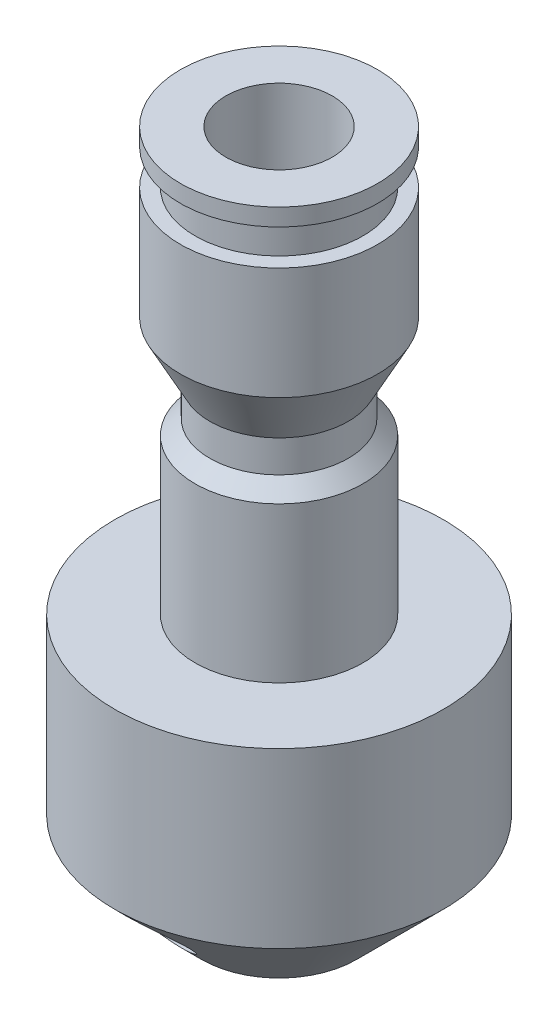
SolidWorks part; units mm, degrees
ref_plane "Front Plane" through (0, 0, 0) normal (0, 0, 1) x (1, 0, 0)
ref_plane "Top Plane" through (0, 0, 0) normal (0, 1, 0) x (1, 0, 0)
ref_plane "Right Plane" through (0, 0, 0) normal (1, 0, 0) x (0, 0, -1)
other "Configuration Table"
sketch "Sketch1" plane through (0, 0, 0) normal (0, 0, 1) x (1, 0, 0)
  line L2 (-8.5, -6.487) -> (-8.5, -9.5097) construction
  line L3 (-4.3412, -6.487) -> (-8.5, -6.487) construction
  line L4 (-4.3412, 1.5327) -> (-4.3412, -6.487) construction
  line L5 (-3.5807, 2.2932) -> (-4.3412, 1.5327) construction
  line L6 (-3.5807, 3.9485) -> (-3.5807, 2.2932) construction
  line L7 (-5.1016, 6.8272) -> (-3.5807, 3.9485) construction
  line L8 (-5.1016, 12.6339) -> (-5.1016, 6.8272) construction
  line L9 (-5.1016, 12.6339) -> (-4.3412, 12.6339) construction
  line L10 (-4.3412, 12.6339) -> (-4.3412, 14.4706) construction
  line L11 (-4.3412, 14.4706) -> (-5.1016, 14.4706) construction
  line L12 (-5.1016, 14.4706) -> (-5.1016, 15.3648) construction
  line L13 (-5.1016, 15.3648) -> (0, 15.3648) construction
  line L16 (-8.5, -6.487) -> (-8.5, -15.4451)
  line L17 (-4.3412, -6.487) -> (-8.5, -6.487)
  line L18 (-4.3412, 1.5327) -> (-4.3412, -6.487)
  line L19 (-3.5807, 2.2932) -> (-4.3412, 1.5327)
  line L20 (-3.5807, 3.9485) -> (-3.5807, 2.2932)
  line L21 (-5.1016, 6.8272) -> (-3.5807, 3.9485)
  line L22 (-5.1016, 12.6339) -> (-5.1016, 6.8272)
  line L23 (-5.1016, 12.6339) -> (-4.3412, 12.6339)
  line L24 (-4.3412, 12.6339) -> (-4.3412, 14.4706)
  line L25 (-4.3412, 14.4706) -> (-5.1016, 14.4706)
  line L26 (-5.1016, 14.4706) -> (-5.1016, 15.3648)
  line L27 (-5.1016, 15.3648) -> (0, 15.3648)
  line L28 (0, 12.6339) -> (0, -12.8923) construction
  line L29 (0, 12.6339) -> (0, -19.9451)
  line L30 (0, 15.3648) -> (0, 12.6339) construction
  line L31 (0, 15.3648) -> (0, 12.6339)
  line L32 (-4, -19.9451) -> (0, -19.9451)
  line L33 (-8.5, -15.4451) -> (-4, -19.9451) construction
  line L34 (-4, -19.9451) -> (-4, -22.0664) construction
  line L35 (-4, -19.9451) -> (-8.5, -15.4451)
  line L36 (-8.5, 0.9336) -> (-8.5, -15.4451) construction
  line L37 (-8.5, -15.4451) -> (-4, -19.9451) construction
revolve "Revolve1" add sketch "Sketch1" angle 360 about L29
sketch "Sketch3" plane through (0, 15.3648, 0) normal (0, 1, 0) x (1, 0, 0)
  circle A0 centre (0, 0) radius 2.75
  dimension "D1" = 5.5
extrude "Cut-Extrude2" cut sketch "Sketch3" against normal blind 4
sketch "Sketch4" plane through (0, -19.9451, 0) normal (0, -1, 0) x (1, 0, 0)
  circle A0 centre (0, 0) radius 4
extrude "Cut-Extrude3" cut sketch "Sketch4" against normal blind 10
sketch "Sketch5" plane through (0, 0, 0) normal (1, 0, 0) x (0, 0, -1)
  line L0 (-8.5, -15.4451) -> (8.5, -15.4451) construction
  line L1 (3.4828, -17.4451) -> (9.1818, -17.4451)
  line L2 (3.4828, -17.4451) -> (3.4828, -15.9451)
  line L3 (3.4828, -15.9451) -> (9.1818, -15.9451)
  line L4 (9.1818, -17.4451) -> (9.1818, -15.9451)
  dimension "D1" = 0.5
  dimension "D2" = 1.5
revolve "Cut-Revolve1" cut sketch "Sketch5" angle 360 about L1
mirror "Mirror1" about plane through (0, 0, 0) normal (0, 0, 1) of "Cut-Revolve1"
